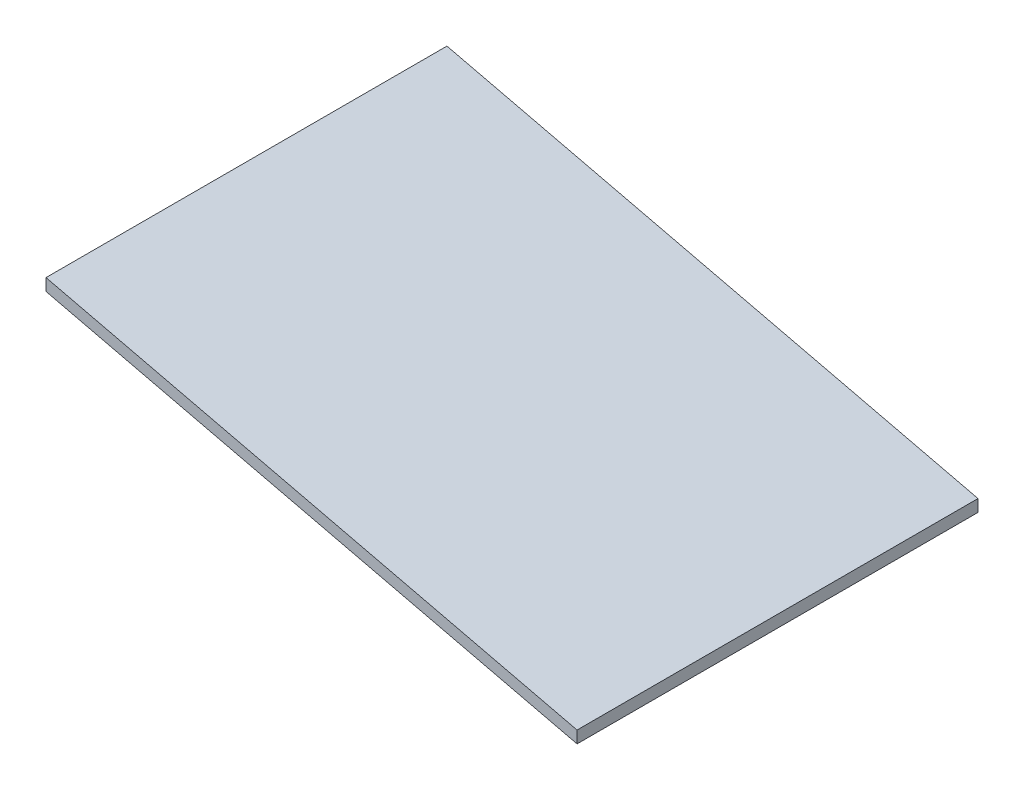
SolidWorks part; units mm, degrees
ref_plane "前视基准面" through (0, 0, 0) normal (0, 0, 1) x (1, 0, 0)
ref_plane "上视基准面" through (0, 0, 0) normal (0, 1, 0) x (1, 0, 0)
ref_plane "右视基准面" through (0, 0, 0) normal (1, 0, 0) x (0, 0, -1)
sketch "草图1" plane through (0, 0, 0) normal (0, 0, 1) x (1, 0, 0)
  line L0 (0, 0) -> (1324.5, -315)
  line L1 (1324.5, -315) -> (1324.5, -345)
  line L2 (1324.5, -345) -> (0, -30)
  line L3 (0, -30) -> (0, 0)
extrude "凸台-拉伸1" add sketch "草图1" along normal blind 1000
